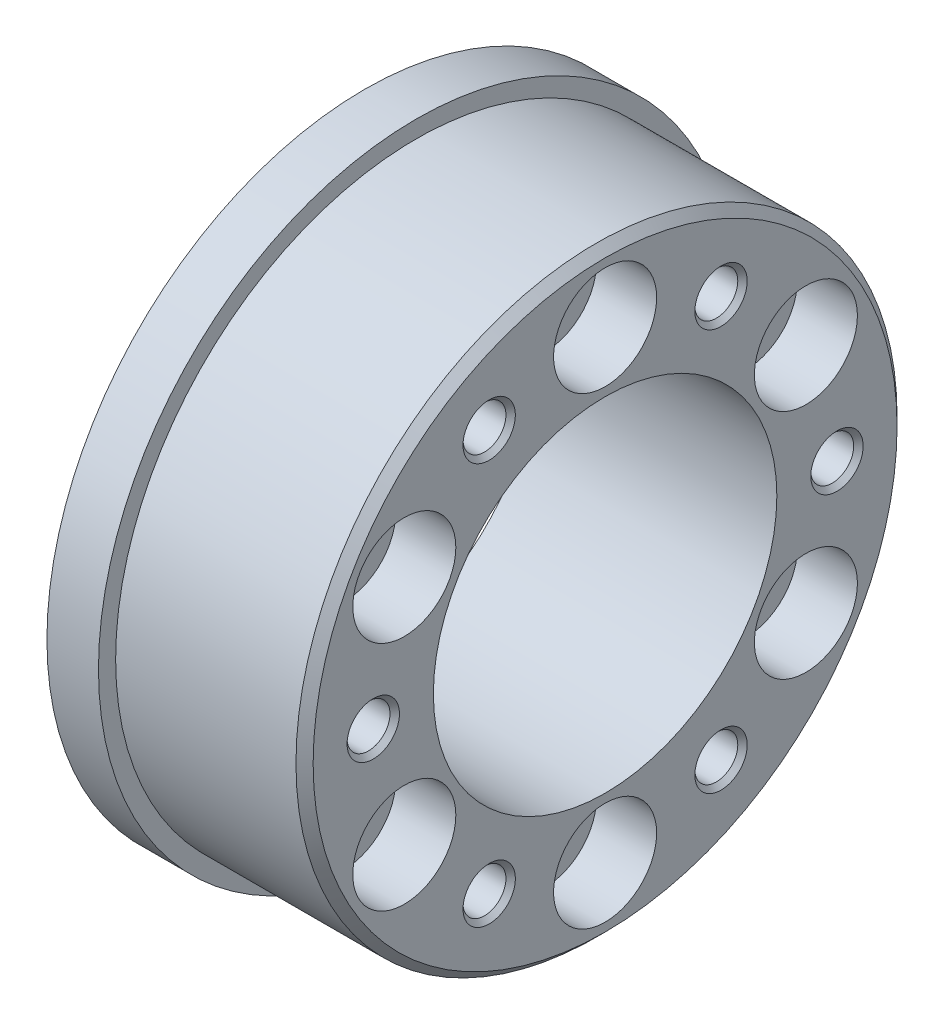
from build123d import *

# Parameters (mm, degrees)
SKETCH_2_R                   = 1.6
CUT_EXTRUDE_1_DEPTH          = 30.67322025
CHAMFER_1_SIZE               = 0.5
SKETCH_3_R                   = 3
CUT_EXTRUDE_2_DEPTH          = 3.5
HOLE_WIZARD_M3_1_D           = 2.5
HOLE_WIZARD_M3_1_CSINK_D     = 3.05
HOLE_WIZARD_M3_1_CSINK_ANGLE = 90


with BuildPart() as part:
    # 草图1 → 旋转1 (revolve)
    with BuildSketch(Plane(origin=(0, 0, 0), x_dir=(1, 0, 0), z_dir=(0, 1, 0)), mode=Mode.PRIVATE) as revolve_1_sk:
        Polygon((0, 18.5), (3, 18.5), (3, 17.5), (14, 17.5), (14, 10), (0, 10), align=None)
    revolve(revolve_1_sk.sketch.rotate(Axis((-415.591715209, 0, 0), (1, 0, 0)), 180), axis=Axis((-415.591715209, 0, 0), (1, 0, 0)))

    # 草图2 → 切除-拉伸1 (cut, through all)
    with BuildSketch(Plane(origin=(14, 0, 0), x_dir=(0, 0, -1), z_dir=(1, 0, 0))):
        with Locations((0, 13.5)):
            Circle(SKETCH_2_R)
        with Locations((11.691342951, 6.75)):
            Circle(SKETCH_2_R)
        with Locations((11.691342951, -6.75)):
            Circle(SKETCH_2_R)
        with Locations((0, -13.5)):
            Circle(SKETCH_2_R)
        with Locations((-11.691342951, -6.75)):
            Circle(SKETCH_2_R)
        with Locations((-11.691342951, 6.75)):
            Circle(SKETCH_2_R)
    extrude(amount=-CUT_EXTRUDE_1_DEPTH, mode=Mode.SUBTRACT)

    # 倒角1
    chamfer_1_edges = [part.edges().sort_by_distance(p)[0] for p in [
        (14, 0, -17.5),
    ]]
    chamfer(chamfer_1_edges, length=CHAMFER_1_SIZE)

    # 草图3 → 切除-拉伸2 (cut)
    with BuildSketch(Plane(origin=(14, 0, 0), x_dir=(0, 0, -1), z_dir=(1, 0, 0))):
        with Locations((0, 13.5)):
            Circle(SKETCH_3_R)
        with Locations((11.691342951, 6.75)):
            Circle(SKETCH_3_R)
        with Locations((11.691342951, -6.75)):
            Circle(SKETCH_3_R)
        with Locations((0, -13.5)):
            Circle(SKETCH_3_R)
        with Locations((-11.691342951, -6.75)):
            Circle(SKETCH_3_R)
        with Locations((-11.691342951, 6.75)):
            Circle(SKETCH_3_R)
    extrude(amount=-CUT_EXTRUDE_2_DEPTH, mode=Mode.SUBTRACT)

    # M3 螺纹孔1 (through all)
    with Locations(Plane(origin=(14, 0, 0), x_dir=(0, 0, -1), z_dir=(1, 0, 0))):
        with Locations((-6.75, 11.691342951), (6.75, 11.691342951), (13.5, 0), (6.75, -11.691342951), (-6.75, -11.691342951), (-13.5, 0)):
            CounterSinkHole(HOLE_WIZARD_M3_1_D / 2, HOLE_WIZARD_M3_1_CSINK_D / 2, counter_sink_angle=HOLE_WIZARD_M3_1_CSINK_ANGLE)


solid = part.part
